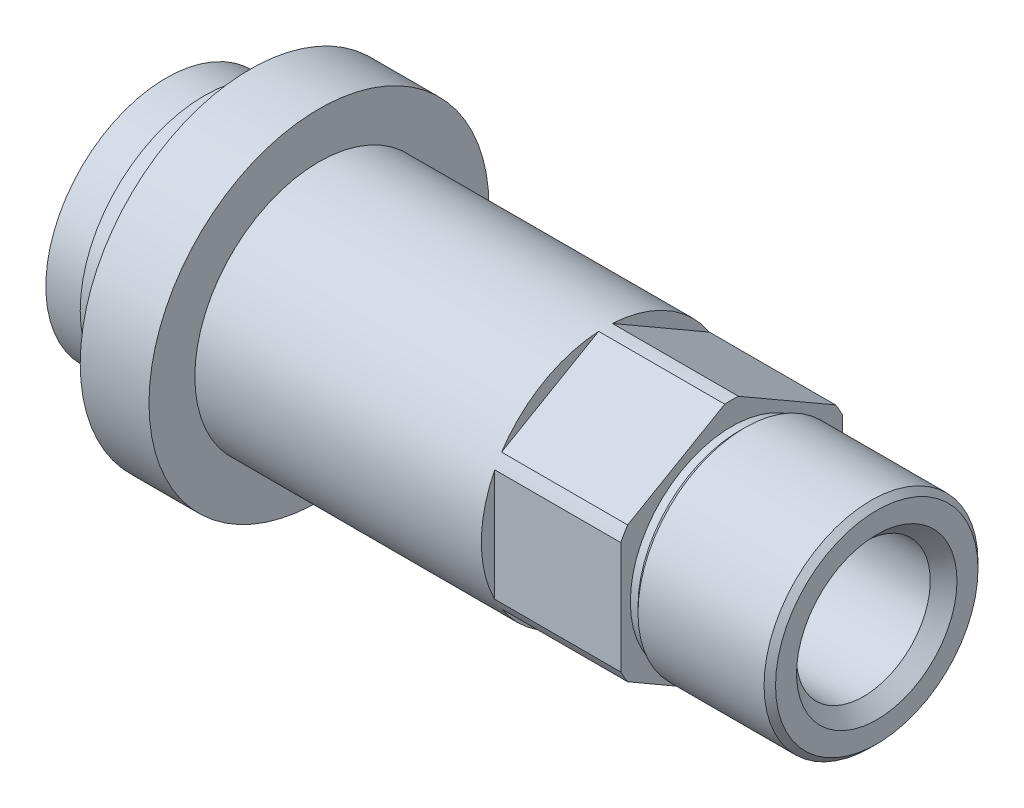
SolidWorks part; units mm, degrees
ref_plane "Front Plane" through (0, 0, 0) normal (0, 0, 1) x (1, 0, 0)
ref_plane "Top Plane" through (0, 0, 0) normal (0, 1, 0) x (1, 0, 0)
ref_plane "Right Plane" through (0, 0, 0) normal (1, 0, 0) x (0, 0, -1)
sketch "Sketch1" plane through (0, 0, 0) normal (0, 0, 1) x (1, 0, 0)
  line L0 (-36, 26.5) -> (-34.5, 28)
  line L1 (0, 0) -> (-38, 0)
  line L2 (0, 0) -> (0, 28)
  line L3 (0, 28) -> (-38, 28)
  line L4 (-38, 26.5) -> (-38, 28)
  line L5 (-38, 0) -> (-146, 0)
  line L6 (-38, 26.5) -> (-38, 32.5)
  line L7 (-38, 32.5) -> (-146, 32.5)
  line L8 (-146, 0) -> (-146, 32.5) construction
  line L9 (-146, 0) -> (-164, 0)
  line L10 (-146, 32.5) -> (-146, 44.5)
  line L11 (-146, 44.5) -> (-164, 44.5)
  line L12 (-164, 32.5) -> (-164, 44.5)
  line L13 (-164, 0) -> (-176, 0)
  line L14 (-164, 0) -> (-164, 32.5) construction
  line L15 (-164, 32.5) -> (-176, 32.5)
  line L16 (-176, 31.5) -> (-176, 32.5)
  line L17 (-176, 0) -> (-186, 0)
  line L18 (-176, 0) -> (-176, 31.5) construction
  line L19 (-176, 31.5) -> (-186, 31.5)
  line L20 (-186, 0) -> (-186, 31.5)
  line L21 (-38, 28) -> (-36, 28)
  line L22 (-38, 28) -> (-38, 26.5)
  line L23 (-38, 26.5) -> (-36, 26.5)
  line L24 (-36, 28) -> (-36, 26.5) construction
  line L25 (-38, 0) -> (-38, 26.5) construction
  line L26 (-38, 0) -> (-38, 26.5) construction
  line L27 (-146, 0) -> (-146, 32.5) construction
  line L28 (-164, 0) -> (-164, 32.5) construction
  line L29 (-176, 0) -> (-176, 31.5) construction
  dimension "D1" = 28
  dimension "D2" = 38
  dimension "D3" = 32.5
  dimension "D4" = 146
  dimension "D5" = 44.5
  dimension "D6" = 18
  dimension "D7" = 32.5
  dimension "D8" = 12
  dimension "D9" = 31.5
  dimension "D10" = 186
  dimension "D11" = 26.5
  dimension "D12" = 45
  dimension "D13" = 1.5
  dimension "D14" = 3.5
revolve "Revolve1" add sketch "Sketch1" angle 360 about L1
chamfer "Chamfer1" distance 1.5 angle 45 1 edges at (0, 0, -28)
sketch "Sketch2" plane through (-38, 0, 0) normal (1, 0, 0) x (0, 0, -1)
  line L1 (0, -33.4863) -> (29, -16.7432)
  line L2 (29, -16.7432) -> (29, 16.7432)
  line L3 (29, 16.7432) -> (0, 33.4863)
  line L4 (0, 33.4863) -> (-29, 16.7432)
  line L5 (-29, 16.7432) -> (-29, -16.7432)
  line L6 (-29, -16.7432) -> (0, -33.4863)
  circle A0 centre (0, 0) radius 29 construction
  circle A2 centre (0, 0) radius 32.5
  circle A3 centre (0, 0) radius 32.5
  circle M1 centre (0, 0) radius 32.5
  dimension "D1" = 58
  dimension "D2" = 0
extrude "Cut-Extrude1" cut sketch "Sketch2" against normal blind 71 from surface at 38 contours L3 M1 starting at face at (0, 0, -26.5)
pattern_circular "CirPattern1" count 6 over 360 about axis through (0, 0, 0) along (1, 0, 0) of "Cut-Extrude1"
sketch "Sketch4" plane through (0, 0, 0) normal (0, 0, 1) x (1, 0, 0)
  line L0 (-186, 31.5) -> (-186, -31.5) construction
  line L1 (0, 0) -> (-70, 0)
  line L2 (0, 0) -> (0, 17.5)
  line L3 (0, 17.5) -> (-66.5, 17.5)
  line L4 (-70, 0) -> (-70, 17.5) construction
  line L5 (-70, 0) -> (-186, 0)
  line L6 (-70, 17.5) -> (-70, 21) construction
  line L7 (-70, 21) -> (-186, 21)
  line L8 (-186, 0) -> (-186, 21)
  line L9 (-70, 21) -> (-66.5, 17.5)
  line L10 (-70, 0) -> (-70, 17.5) construction
  line L11 (-66.5, 17.5) -> (-70, 17.5) construction
  dimension "D1" = 21
  dimension "D2" = 70
  dimension "D3" = 3.5
  dimension "D4" = 45
revolve "Cut-Revolve2" cut sketch "Sketch4" angle 360 about L1
chamfer "Chamfer3" distance 3.5 angle 45 1 edges at (0, 17.5, 0)
